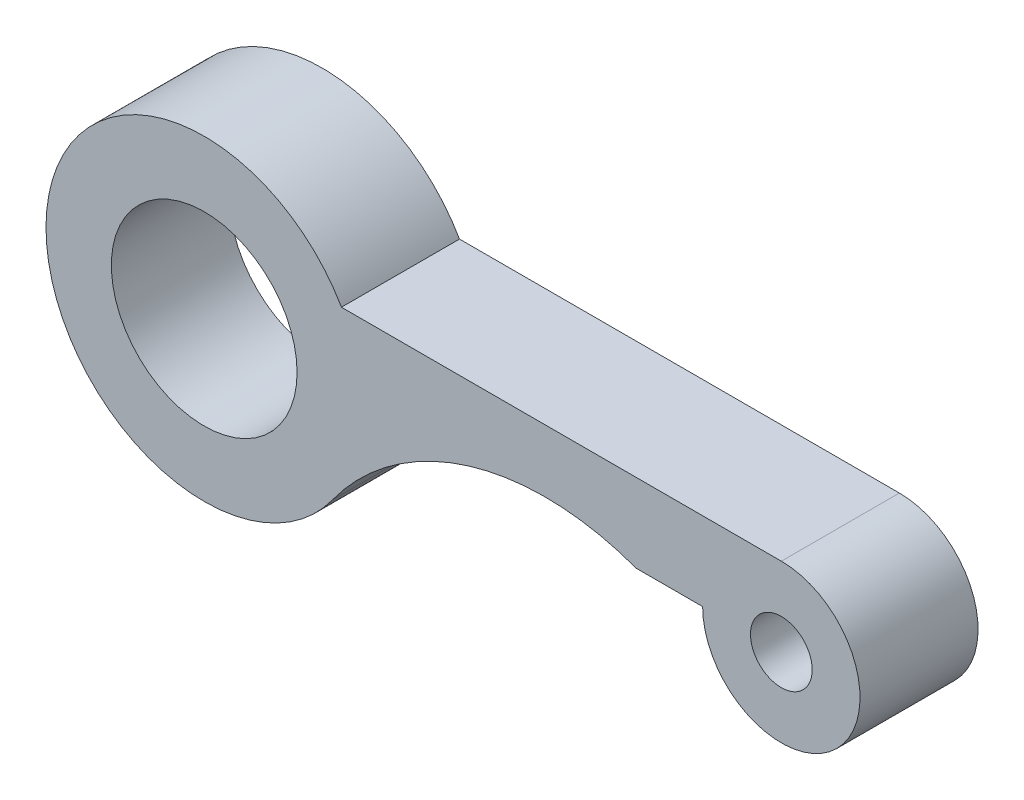
SolidWorks part; units mm, degrees
material "1060 合金"
ref_plane "前视基准面" through (0, 0, 0) normal (0, 0, 1) x (1, 0, 0)
ref_plane "上视基准面" through (0, 0, 0) normal (0, 1, 0) x (1, 0, 0)
ref_plane "右视基准面" through (0, 0, 0) normal (1, 0, 0) x (0, 0, -1)
sketch "草图1" plane through (0, 0, 0) normal (0, 0, 1) x (1, 0, 0)
  line L0 (6.0311, 0) -> (22, 0) construction
  line L3 (22, 3) -> (5.2321, 3)
  circle A0 centre (0, 0) radius 6.0311
  circle A1 centre (0, 0) radius 3.54
  circle A3 centre (22, 0) radius 1.176
  circle A8 centre (22, 0) radius 3
  arc A9 (19.9231, -2.1648) -> (4.8908, -3.5292) centre (12.9999, -9.3808) ccw
  dimension "D1" = 22
  dimension "D2" = 20
extrude "凸台-拉伸1" add sketch "草图1" along normal blind 4.5
